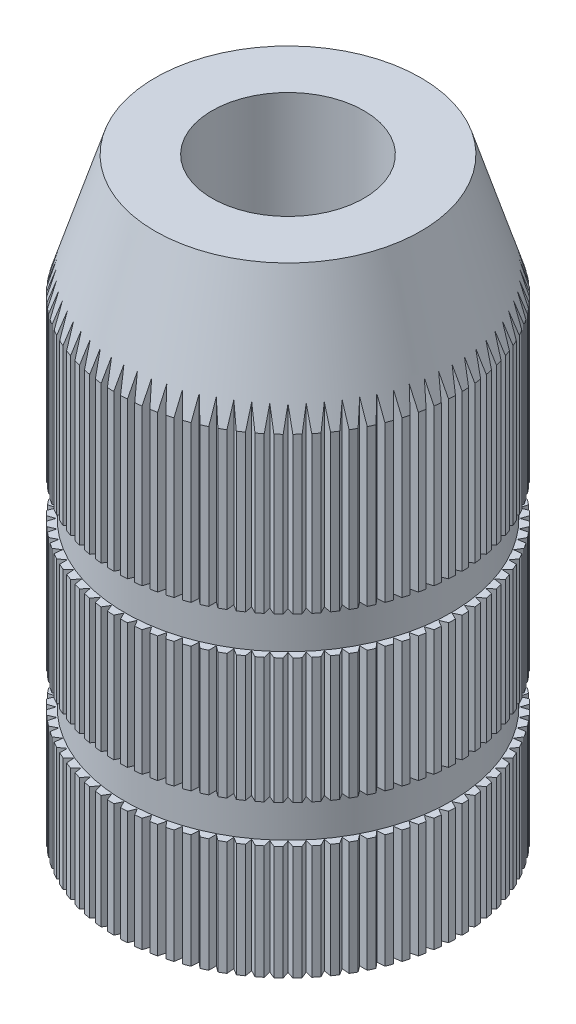
SolidWorks part; units mm, degrees
material "铜H591"
ref_plane "前视基准面" through (0, 0, 0) normal (0, 0, 1) x (1, 0, 0)
ref_plane "上视基准面" through (0, 0, 0) normal (0, 1, 0) x (1, 0, 0)
ref_plane "右视基准面" through (0, 0, 0) normal (1, 0, 0) x (0, 0, -1)
sketch "草图1" plane through (0, 0, 0) normal (0, 0, 1) x (1, 0, 0)
  line L0 (0, 0) -> (0, 8.7643) construction
  line L1 (-2.25, 0) -> (-2.25, 6.2)
  line L2 (-2.25, 6.2) -> (-1.75, 7.8)
  line L3 (-1.75, 7.8) -> (-1, 7.8)
  line L4 (-1, 7.8) -> (-1, 0.2)
  line L7 (-1.2, 0) -> (-2.25, 0)
  line L8 (-1, 0.2) -> (-1.2, 0)
  point P13 (-1, 0)
  dimension "D1" = 4.5
  dimension "D2" = 2
  dimension "D3" = 7.8
  dimension "D4" = 3.5
  dimension "D5" = 6.2
revolve "旋转1" add sketch "草图1" angle 360 about L0
sketch "草图2" plane through (0, 0, 0) normal (0, -1, 0) x (1, 0, 0)
  line L0 (-2.3447, 0) -> (2.3447, 0) construction
  line L1 (-2.26, 0.05) -> (-2.26, -0.05)
  line L2 (-2.26, -0.05) -> (-2.16, 0)
  line L3 (-2.16, 0) -> (-2.26, 0.05)
  circle A0 centre (0, 0) radius 2.25 construction
  point P3 (0, 0)
  dimension "D1" = 0.01
  dimension "D2" = 0.1
  dimension "D3" = 0.1
extrude "切除-拉伸1" cut sketch "草图2" against normal blind 10
pattern_circular "阵列(圆周)1" count 80 over 360 about axis through (0, 0, 0) along (0, 1, 0) of "切除-拉伸1"
sketch "草图3" plane through (0, 0, 0) normal (0, 0, 1) x (1, 0, 0)
  line L0 (0, 0) -> (0, 8.8117) construction
  line L1 (-2.4538, 2) -> (-2.15, 2)
  line L2 (-2.4538, 2) -> (-2.4538, 1.5)
  line L3 (-2.4538, 1.5) -> (-2.15, 1.5)
  line L4 (-2.15, 2) -> (-2.15, 1.5)
  line L6 (-2.4538, 4.15) -> (-2.15, 4.15)
  line L7 (-2.4538, 4.15) -> (-2.4538, 3.65)
  line L8 (-2.4538, 3.65) -> (-2.15, 3.65)
  line L9 (-2.15, 4.15) -> (-2.15, 3.65)
  dimension "D1" = 1.5
  dimension "D2" = 4.3
  dimension "D3" = 0.5
  dimension "D4" = 1.65
  dimension "D5" = 0.5
revolve "切除-旋转1" cut sketch "草图3" angle 360 about L0
